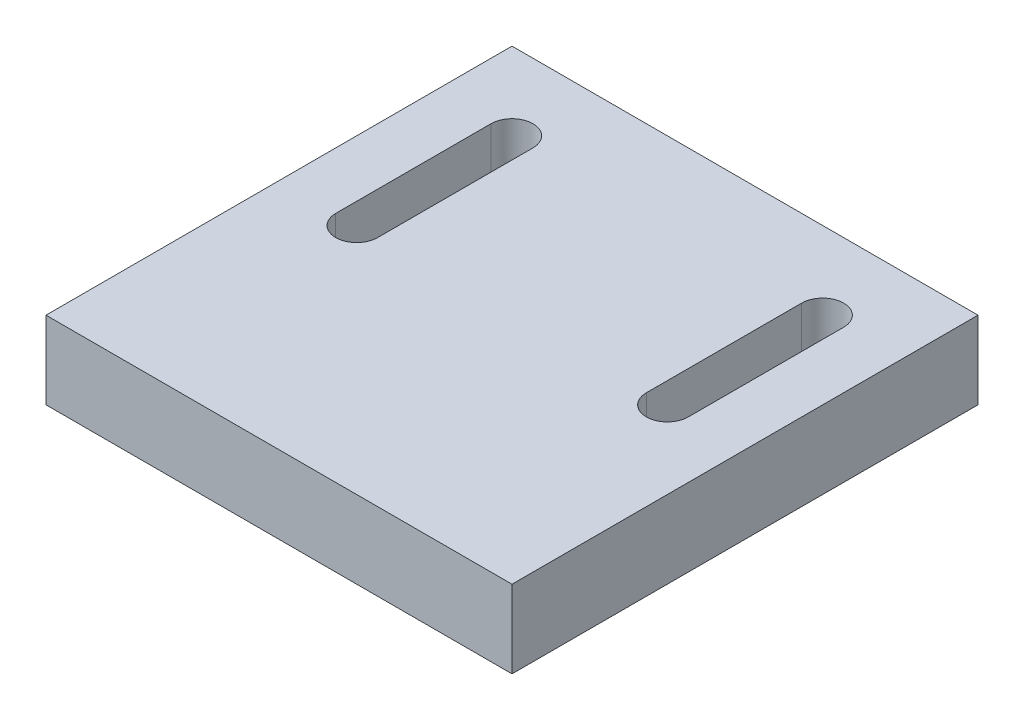
SolidWorks part; units mm, degrees
ref_plane "Front Plane" through (0, 0, 0) normal (0, 0, 1) x (1, 0, 0)
ref_plane "Top Plane" through (0, 0, 0) normal (0, 1, 0) x (1, 0, 0)
ref_plane "Right Plane" through (0, 0, 0) normal (1, 0, 0) x (0, 0, -1)
sketch "Sketch1" plane through (0, 0, 0) normal (0, 1, 0) x (1, 0, 0)
  line L1 (-30, 30) -> (30, 30)
  line L2 (-30, 30) -> (-30, -30)
  line L3 (-30, -30) -> (30, -30)
  line L4 (30, 30) -> (30, -30)
  line L5 (-30, 30) -> (30, -30) construction
  line L6 (-30, -30) -> (30, 30) construction
  point P0 (0, 0)
  dimension "D1" = 60
  dimension "D2" = 60
extrude "Boss-Extrude1" add sketch "Sketch1" along normal blind 10
sketch "Sketch2" plane through (0, 10, 0) normal (0, 1, 0) x (1, 0, 0)
  line L0 (20, 0) -> (20, 20) construction
  line L1 (17.3, 0) -> (17.3, 20)
  line L2 (22.7, 0) -> (22.7, 20)
  line L3 (30, 30) -> (-30, 30) construction
  arc A0 (17.3, 0) -> (22.7, 0) centre (20, 0) ccw
  arc A1 (22.7, 20) -> (17.3, 20) centre (20, 20) ccw
  point P2 (20, 10)
  dimension "D1" = 5.4
  dimension "D2" = 20
  dimension "D3" = 20
  dimension "D4" = 20
extrude "Cut-Extrude1" cut sketch "Sketch2" against normal through all
mirror "Mirror1" about plane through (0, 0, 0) normal (1, 0, 0) of "Cut-Extrude1"
